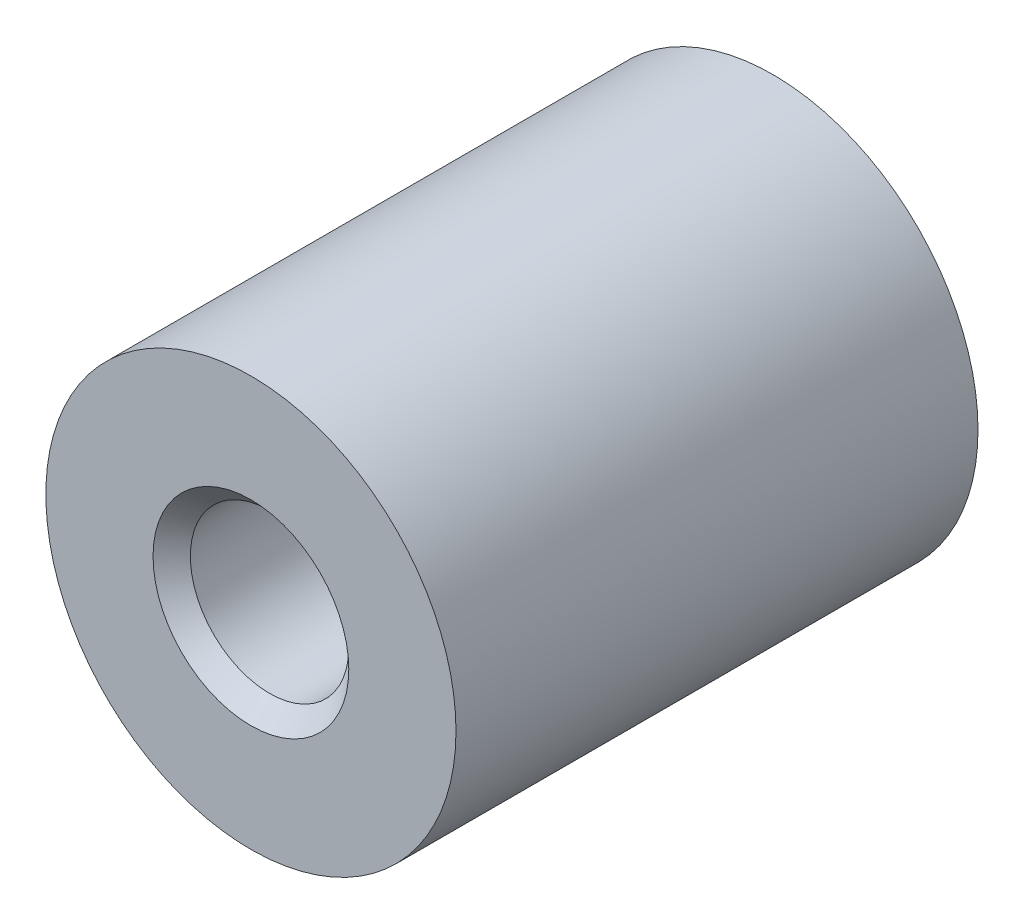
from build123d import *

# Parameters (mm, degrees)
SKETCH1_R           = 11
BOSS_EXTRUDE1_DEPTH = 28
SKETCH2_R           = 4.25
CUT_EXTRUDE1_DEPTH  = 38
CHAMFER1_SIZE       = 1


with BuildPart() as part:
    # Sketch1 → Boss-Extrude1 (new body)
    with BuildSketch(Plane.XY):
        Circle(SKETCH1_R)
    extrude(amount=BOSS_EXTRUDE1_DEPTH)

    # Sketch2 → Cut-Extrude1 (cut)
    with BuildSketch(Plane.XY.offset(28)):
        Circle(SKETCH2_R)
    extrude(amount=-CUT_EXTRUDE1_DEPTH, mode=Mode.SUBTRACT)

    # Chamfer1
    chamfer1_edges = [part.edges().sort_by_distance(p)[0] for p in [
        (-4.25, 0, 28),
    ]]
    chamfer(chamfer1_edges, length=CHAMFER1_SIZE)


solid = part.part
